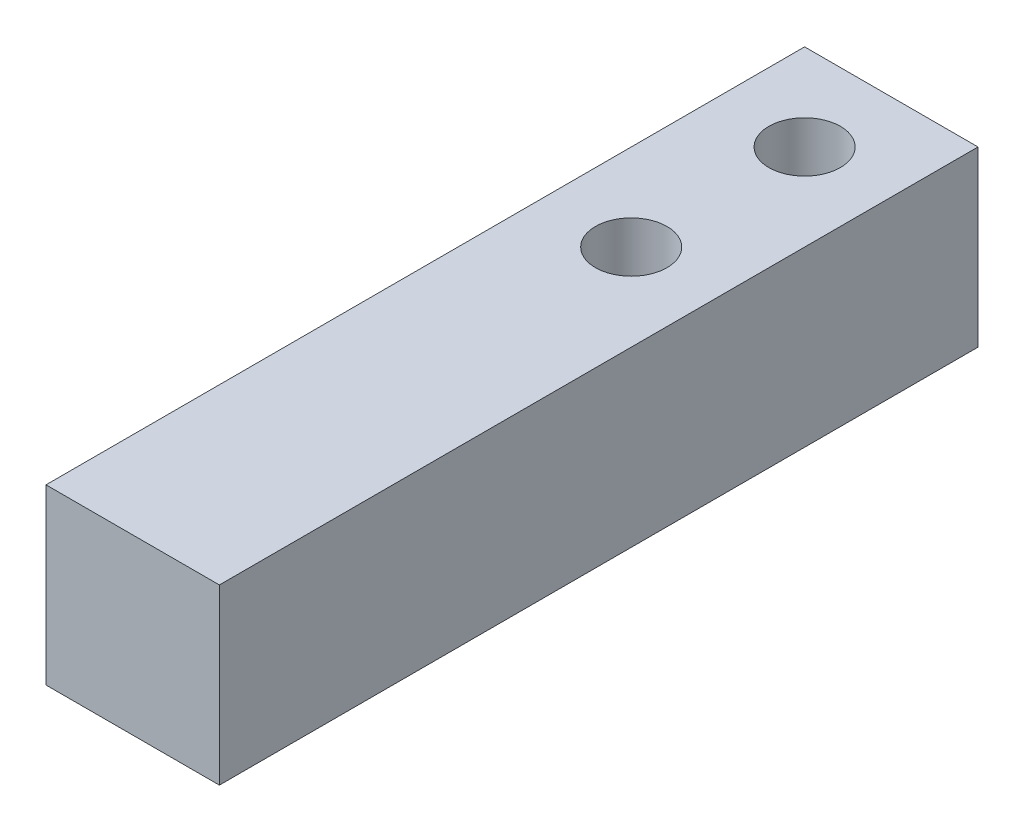
SolidWorks part; units mm, degrees
ref_plane "前视基准面" through (0, 0, 0) normal (0, 0, 1) x (1, 0, 0)
ref_plane "上视基准面" through (0, 0, 0) normal (0, 1, 0) x (1, 0, 0)
ref_plane "右视基准面" through (0, 0, 0) normal (1, 0, 0) x (0, 0, -1)
sketch "草图1" plane through (0, 0, 0) normal (0, 0, 1) x (1, 0, 0)
  line L1 (-4, 4) -> (4, 4)
  line L2 (-4, 4) -> (-4, -4)
  line L3 (-4, -4) -> (4, -4)
  line L4 (4, 4) -> (4, -4)
  line L5 (-4, 4) -> (4, -4) construction
  line L6 (-4, -4) -> (4, 4) construction
  point P0 (0, 0)
  dimension "D1" = 8
  dimension "D2" = 8
extrude "凸台-拉伸1" add sketch "草图1" along normal blind 35
hole_wizard "M4 螺纹孔1" positions "草图5" profile "草图4" tap size "M4" standard "Iso" end condition through all
sketch "草图5" plane through (0, -4, 0) normal (0, -1, 0) x (-1, 0, 0)
  line L0 (0, 0) -> (0, -15.8834) construction
  line L2 (4, 0) -> (-4, 0) construction
  point P0 (0, -12)
  point P2 (0, -4)
  dimension "D1" = 4
  dimension "D2" = 12
sketch "草图4" plane through (0, -4, 12) normal (1, 0, 0) x (0, 0, -1)
  line L0 (0, 0) -> (0, 8)
  line L1 (0, 8) -> (1.65, 8)
  line L2 (1.65, 8) -> (1.65, 0)
  line L5 (1.65, 0) -> (0, 0)
  line L11 (0, -6.35) -> (0, 107.95) construction
  dimension "通孔螺纹孔钻头直径" = 3.3
  dimension "通孔螺纹孔钻头深度" = 8
cosmetic thread "孔螺蚊线1"
cosmetic thread "孔螺蚊线2"
